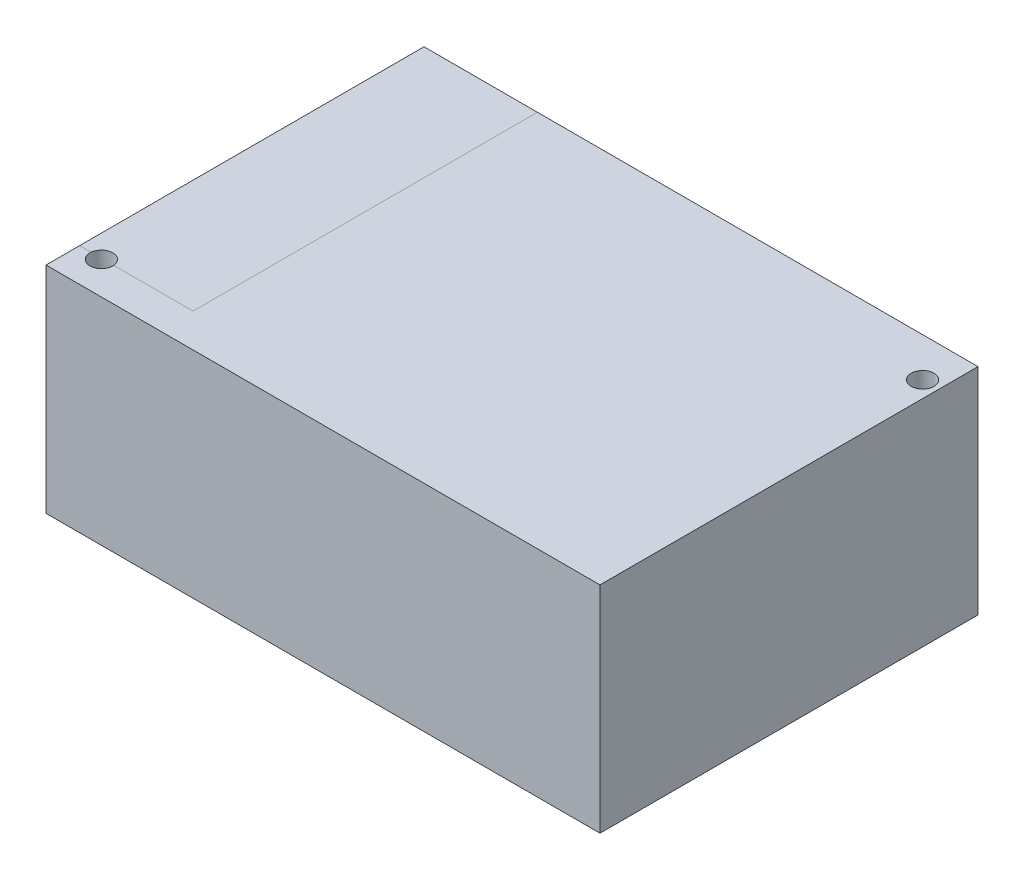
from build123d import *

# Parameters (mm, degrees)
SKETCH_1_W              = 85
SKETCH_1_H              = 58
EXTRUDE_1_DEPTH         = 33
HOLE_WIZARD_3_5_3_5_1_D = 3.5


with BuildPart() as part:
    # 草图1 → 凸台-拉伸1 (new body)
    with BuildSketch(Plane(origin=(0, 0, 0), x_dir=(1, 0, 0), z_dir=(0, 1, 0))):
        Rectangle(SKETCH_1_W, SKETCH_1_H)
    extrude(amount=EXTRUDE_1_DEPTH)

    # Ø3.5 (3.5) 直径孔1 (through all)
    with Locations(Plane(origin=(0, 0, 0), x_dir=(-1, 0, 0), z_dir=(0, -1, 0))):
        with Locations((39, -24), (-40, 23)):
            Hole(HOLE_WIZARD_3_5_3_5_1_D / 2)


solid = part.part
